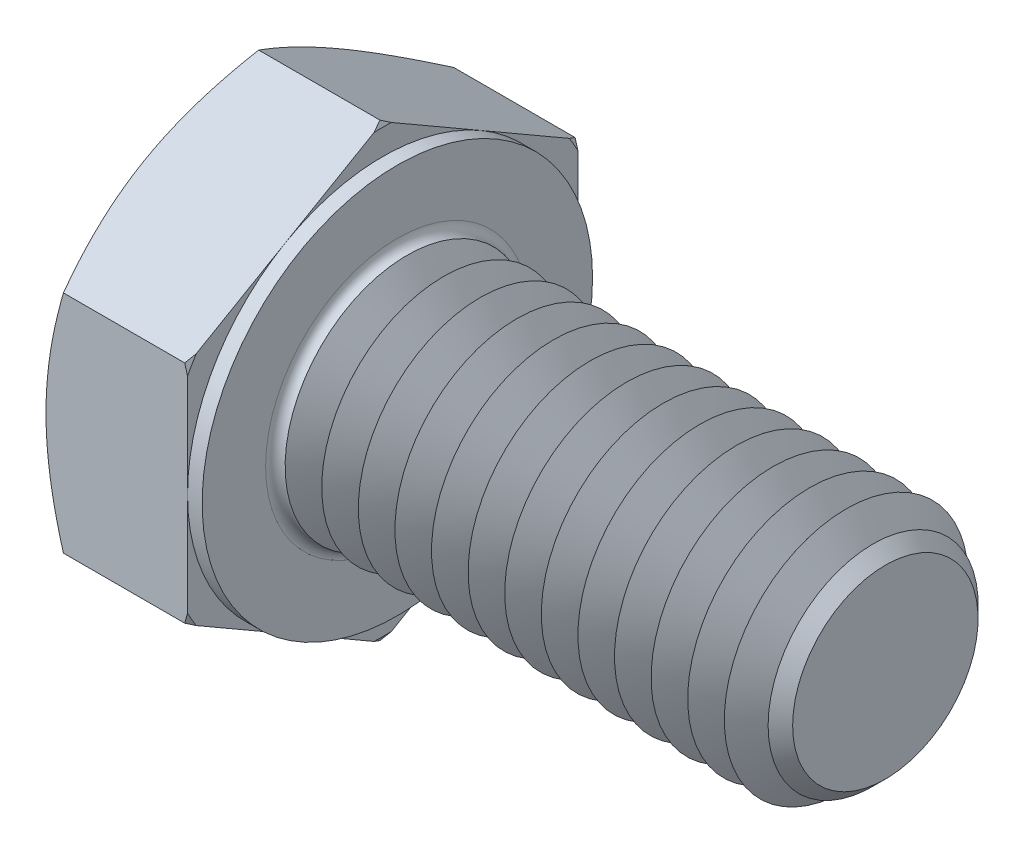
SolidWorks part; units mm, degrees
extrude "Boss-Extrude" add sketch "Sketch1" along normal blind 6.4
sketch "Sketch1" plane through (0, 0, 0) normal (1, 0, 0) x (0, 0, -1)
  line L0 (8, 4.6188) -> (8, -4.6188)
  line L1 (-8, 4.6188) -> (-8, -4.6188)
  line L2 (8, -4.6188) -> (0, -9.2376)
  line L3 (0, -9.2376) -> (-8, -4.6188)
  line L4 (8, 4.6188) -> (0, 9.2376)
  line L5 (0, 9.2376) -> (-8, 4.6188)
revolve "Cut-Revolve1" cut sketch "Sketch3" angle 360 about L6
sketch "Sketch3" plane through (0, 0, 0) normal (0, 0, 1) x (1, 0, 0)
  line L0 (0, 8) -> (3.6013, 14.2376)
  line L1 (0, 9.2376) -> (0, 4.6188) construction
  line L2 (3.6013, 14.2376) -> (3.6013, 19.2376)
  line L3 (3.6013, 19.2376) -> (-10, 19.2376)
  line L4 (-10, 19.2376) -> (-10, 8)
  line L5 (-10, 8) -> (0, 8)
  line L6 (0, 0) -> (99.06, 0) construction
  line L7 (6.4, 9.2376) -> (0, 9.2376) construction
revolve "Boss-Revolve1" add sketch "Sketch2" angle 360 about L7
sketch "Sketch2" plane through (0, 0, 0) normal (0, 0, 1) x (1, 0, 0)
  line L0 (0, 4.6188) -> (0, -4.6188) construction
  line L1 (0, 0) -> (26.4, 0)
  line L2 (0, 0) -> (0, 5)
  line L3 (0, 5) -> (26.4, 5)
  line L4 (26.4, 0) -> (26.4, 3.701)
  line L5 (6.4, 9.2376) -> (6.4, 4.6188) construction
  line L7 (0, 0) -> (96.52, 0) construction
  line L8 (26.4, -3.701) -> (90.335, -5) construction
  line L9 (0, -5) -> (90.335, -5) construction
  line L10 (7.9, 15.24) -> (7.9, -1.27) construction
  line L11 (6.4, 15.24) -> (6.4, -1.27) construction
  line L12 (6.4, 4.6188) -> (6.4, -4.6188) construction
  line L14 (26.4, 5) -> (26.4, 3.701)
  dimension "l" = 20
  dimension "m" = 10
  dimension "Minor_dia" = 7.402
  dimension "p" = 1.5
  dimension "h" = 20
cosmetic thread "Helix1" parameters "Thread_length"=18.5, "Thread_minor"=7.402
ref_plane "Front Plane" through (0, 0, 0) normal (0, 0, 1) x (1, 0, 0)
ref_plane "Top Plane" through (0, 0, 0) normal (0, 1, 0) x (1, 0, 0)
ref_plane "Right Plane" through (0, 0, 0) normal (1, 0, 0) x (0, 0, -1)
sketch "Sketch5" plane through (0, 0, 0) normal (0, 0, 1) x (1, 0, 0)
  line L0 (6.4, 8) -> (2.7987, 14.2376)
  line L1 (6.4, 9.2376) -> (6.4, 4.6188) construction
  line L2 (2.7987, 14.2376) -> (2.7987, 19.2376)
  line L3 (2.7987, 19.2376) -> (12.7987, 19.2376)
  line L4 (12.7987, 19.2376) -> (12.7987, 8)
  line L5 (12.7987, 8) -> (6.4, 8)
  line L7 (6.4, 9.2376) -> (0.7145, 9.2376) construction
  line L8 (0, 0) -> (99.06, 0) construction
  line L9 (0, 0) -> (99.06, 0) construction
revolve "Cut-Revolve2" cut sketch "Sketch5" angle 360 about L8
sketch "Sketch4" plane through (0, 0, 0) normal (0, 0, 1) x (1, 0, 0)
  line L1 (6.4, 9.2376) -> (6.4, 4.6188) construction
  line L2 (6.4, 8) -> (5.8, 8)
  line L3 (6.4, 8) -> (6.4, 19.2376)
  line L4 (6.4, 19.2376) -> (5.8, 19.2376)
  line L5 (0, 0) -> (95.25, 0) construction
  line L6 (0, 0) -> (96.52, 0) construction
  line L7 (5.8, 8) -> (5.8, 19.2376)
  line L8 (5.6855, 9.2376) -> (0.7145, 9.2376) construction
revolve "Cut-Revolve3" cut sketch "Sketch4" angle 360 about L5
chamfer "Chamfer" distance 1.2 angle 45 1 edges at (26.4, 0, 5)
fillet "Fillet" radius 0.4 1 edges at (6.4, 0, -5)
sketch "Sketch6" plane through (0, 0, 0) normal (0, 0, 1) x (1, 0, 0)
  line L0 (7.55, -3.701) -> (6.8, -5)
  line L1 (7.55, -3.701) -> (8.3, -5)
  line L2 (8.3, -5) -> (8.3, -6.25)
  line L3 (-3.175, 0) -> (5.1513, 0) construction
  line L5 (8.3, -6.25) -> (6.8, -6.25)
  line L6 (6.8, -6.25) -> (6.8, -5)
  arc A0 (6.8, -5) -> (6.4, -5.4) centre (6.8, -5.4) ccw construction
revolve "Cut-Revolve4" cut sketch "Sketch6" angle 360 about L3
pattern_linear "LPattern1" count 13 spacing 1.5 along (1, 0, 0) of "Cut-Revolve4"
equation "\"D3@Sketch1\" = \"s@Sketch1\" / 2"
equation "\"D4@Sketch1\" = \"D3@Sketch1\""
equation "\"D5@Sketch1\" = \"D4@Sketch1\""
equation "\"D1@Sketch3\" = \"s@Sketch1\" / 2"
equation "\"D1@Sketch5\" = \"s@Sketch1\" / 2"
equation "\"Head_ch_ang@Sketch5\" = \"Head_ch_ang@Sketch3\""
equation "\"D1@Sketch4\" = \"s@Sketch1\""
equation "\"Diameter@Sketch6\" = \"m@Sketch2\""
equation "\"Overcut@Sketch6\" = \"m@Sketch2\" * 1.25"
equation "\"Minor_dia@Sketch2\" = \"m@Sketch2\"-\"p@Sketch2\" * 1.732"
equation "\"Thread_minor@Helix1\" = \"Minor_dia@Sketch2\""
equation "\"Thread_minor@Sketch6\" = \"Minor_dia@Sketch2\""
equation "\"D1@Chamfer\" = \"p@Sketch2\"*0.8"
equation "\"Thread_length@Helix1\" = \"l@Sketch2\" - \"p@Sketch2\""
equation "\"Num_threads@LPattern1\" = \"l@Sketch2\" / \"p@Sketch2\""
